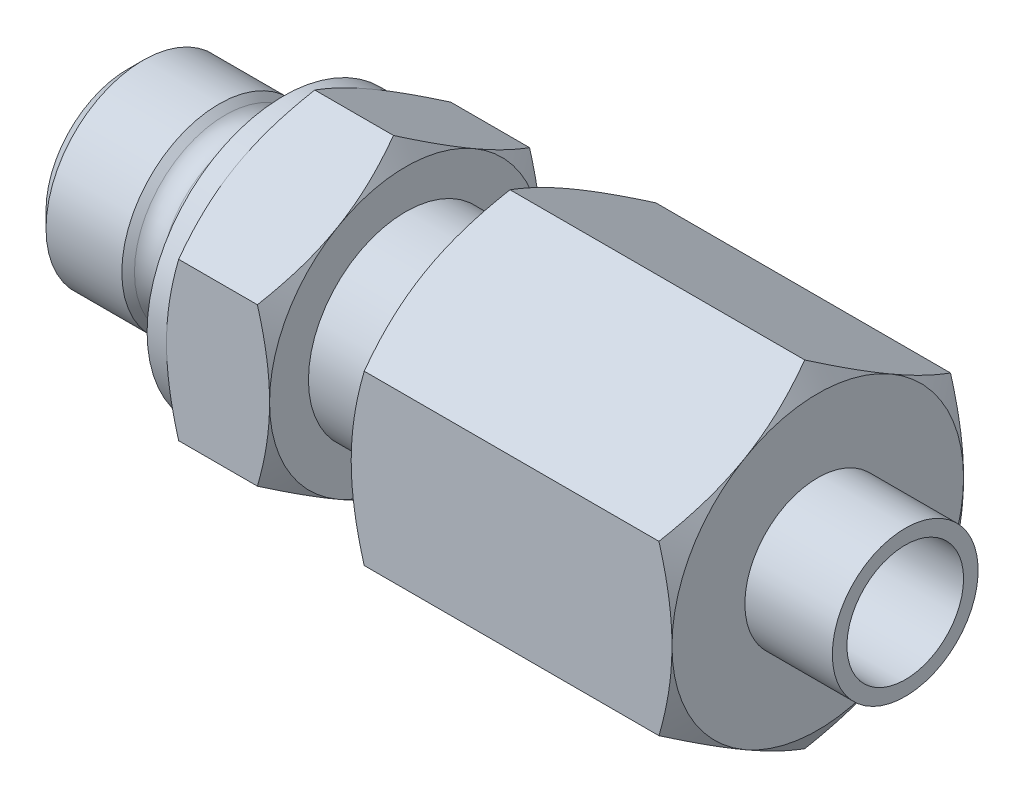
SolidWorks part; units mm, degrees
material "镀铬不锈钢"
ref_plane "前视基准面" through (0, 0, 0) normal (0, 0, 1) x (1, 0, 0)
ref_plane "上视基准面" through (0, 0, 0) normal (0, 1, 0) x (1, 0, 0)
ref_plane "右视基准面" through (0, 0, 0) normal (1, 0, 0) x (0, 0, -1)
sketch "草图1" plane through (0, 0, 0) normal (0, 0, 1) x (1, 0, 0)
  line L0 (0, 2) -> (0, 4.2)
  line L1 (0, 4.2) -> (5.5, 4.2) construction
  line L2 (6.1193, 4.4601) -> (8, 5.25)
  line L3 (8, 7) -> (9, 7)
  line L4 (0, 2) -> (40, 2)
  line L5 (9, 7) -> (14.3, 7) construction
  line L6 (14.3, 7) -> (14.3, 5) construction
  line L7 (14.3, 5) -> (19, 5)
  line L8 (19, 5) -> (19, 7.5)
  line L9 (19, 7.5) -> (35.5, 7.5)
  line L10 (35.5, 7.5) -> (35.5, 3.75)
  line L11 (35.5, 3.75) -> (40, 3.75)
  line L12 (40, 3.75) -> (40, 2)
  line L13 (9, 7) -> (9, 2) construction
  line L14 (0, 0) -> (30, 0) construction
  line L15 (8, 5.25) -> (8, 7)
  line L16 (30, 0) -> (30, -0.9896) construction
  line L17 (30, -0.9896) -> (14.3, -0.9896) construction
  line L18 (19, 5) -> (32.5, 5) construction
  line L19 (40, 2) -> (51, 2) construction
  line L20 (0, 4.2) -> (0.8, 5)
  line L21 (0.8, 5) -> (4.7, 5)
  line L22 (4.7, 5) -> (5.025, 4.675)
  line L23 (18.6, 5) -> (19.6, 6) construction
  line L24 (19.6, 6) -> (23.5, 6) construction
  line L25 (23.5, 6) -> (24.5, 5) construction
  line L26 (24.5, 5) -> (26.5497, 5) construction
  line L27 (26.5497, 5) -> (30, 2.4) construction
  line L28 (30, 2.4) -> (30, 0) construction
  line L29 (30, 0) -> (30, -2.4) construction
  line L30 (30, -2.4) -> (26.5497, -5) construction
  line L31 (51, 2) -> (54.5, 2) construction
  line L32 (9, 7) -> (14.3, 7)
  line L33 (14.3, 7) -> (14.3, 5)
  arc A0 (5.025, 4.675) -> (6.1193, 4.4601) centre (5.7321, 5.3821) ccw
  dimension "rm" = 1
  dimension "d" = 10
  dimension "l" = 8
  dimension "sm" = 14
  dimension "D4" = 7.5
  dimension "lm10" = 35.5
  dimension "d0" = 4
  dimension "sm1" = 15
  dimension "D5" = 3.9
  dimension "D611" = 45
  dimension "D711" = 45
  dimension "d7" = 8.4
  dimension "b1" = 2.5
  dimension "d8" = 10.5
  dimension "d2" = 10
  dimension "b" = 1
  dimension "d6" = 14
  dimension "lm" = 30
  dimension "l4" = 15.7
  dimension "d1" = 12
  dimension "D21" = 45
  dimension "a" = 74
  dimension "h" = 5.5
  dimension "d3" = 4.8
  dimension "5647lm" = 16.5
  dimension "dm3" = 7.5
  dimension "5647l" = 13.5
  dimension "5646lm" = 11
  dimension "5646hm" = 3.5
revolve "旋转1" add sketch "草图1" angle 360 about L14
cosmetic thread "装饰螺纹线1" parameters "D1"=3.9, "D2"=8.4
sketch "草图2" plane through (14.3, 0, 0) normal (1, 0, 0) x (0, 0, -1)
  line L1 (-7, 4.0415) -> (-7, -4.0415)
  line L2 (-7, -4.0415) -> (0, -8.0829)
  line L3 (0, -8.0829) -> (7, -4.0415)
  line L4 (7, -4.0415) -> (7, 4.0415)
  line L5 (7, 4.0415) -> (0, 8.0829)
  line L6 (0, 8.0829) -> (-7, 4.0415)
  circle A0 centre (0, 0) radius 7 construction
  circle A2 centre (0, 0) radius 2 construction
  circle A3 centre (0, 0) radius 2
  dimension "D1" = 14
sketch "草图3" plane through (35.5, 0, 0) normal (1, 0, 0) x (0, 0, -1)
  line L1 (7.5, -4.3301) -> (7.5, 4.3301)
  line L2 (7.5, 4.3301) -> (0, 8.6603)
  line L3 (0, 8.6603) -> (-7.5, 4.3301)
  line L4 (-7.5, 4.3301) -> (-7.5, -4.3301)
  line L5 (-7.5, -4.3301) -> (0, -8.6603)
  line L6 (0, -8.6603) -> (7.5, -4.3301)
  circle A0 centre (0, 0) radius 7.5 construction
  circle A1 centre (0, 0) radius 2 construction
  circle A2 centre (0, 0) radius 7.5 construction
  circle A3 centre (0, 0) radius 2
extrude "拉伸2" add sketch "草图3" against normal up to vertex (16.5 mm away) up to point (19, 7.5, 0)
extrude "凸台-拉伸1" add sketch "草图2" against normal up to vertex (7 mm away)
sketch "草图4" plane through (0, 0, 0) normal (0, 0, 1) x (1, 0, 0)
  line L0 (9, 7) -> (9.6252, 8.0829)
  line L2 (9.6252, 8.0829) -> (9, 8.0829)
  line L3 (9, 8.0829) -> (9, 7)
  line L4 (14.3, 7) -> (13.6748, 8.0829)
  line L5 (13.6748, 8.0829) -> (14.3, 8.0829)
  line L6 (14.3, 8.0829) -> (14.3, 7)
  line L7 (19, 7.5) -> (19.6699, 8.6603)
  line L8 (19, 8.6603) -> (35.5, 8.6603) construction
  line L9 (19.6699, 8.6603) -> (19, 8.6603)
  line L10 (19, 8.6603) -> (19, 7.5)
  line L11 (35.5, 7.5) -> (34.8301, 8.6603)
  line L12 (34.8301, 8.6603) -> (35.5, 8.6603)
  line L13 (35.5, 8.6603) -> (35.5, 7.5)
  line L14 (0, 0) -> (2.9505, 0) construction
  line L15 (0, 0) -> (30, 0) construction
  line L17 (9, 8.0829) -> (14.3, 8.0829) construction
  dimension "D1" = 30
  dimension "D2" = 30
  dimension "D3" = 30
  dimension "D4" = 30
revolve "切除-旋转1" cut sketch "草图4" angle 360 about L14
sketch "草图6" plane through (40, 0, 0) normal (1, 0, 0) x (0, 0, -1)
  circle A0 centre (0, 0) radius 3
  dimension "D0" = 6
extrude "切除-拉伸1" cut sketch "草图6" against normal up to vertex (10 mm away) up to point (30, 2.4, 0)
